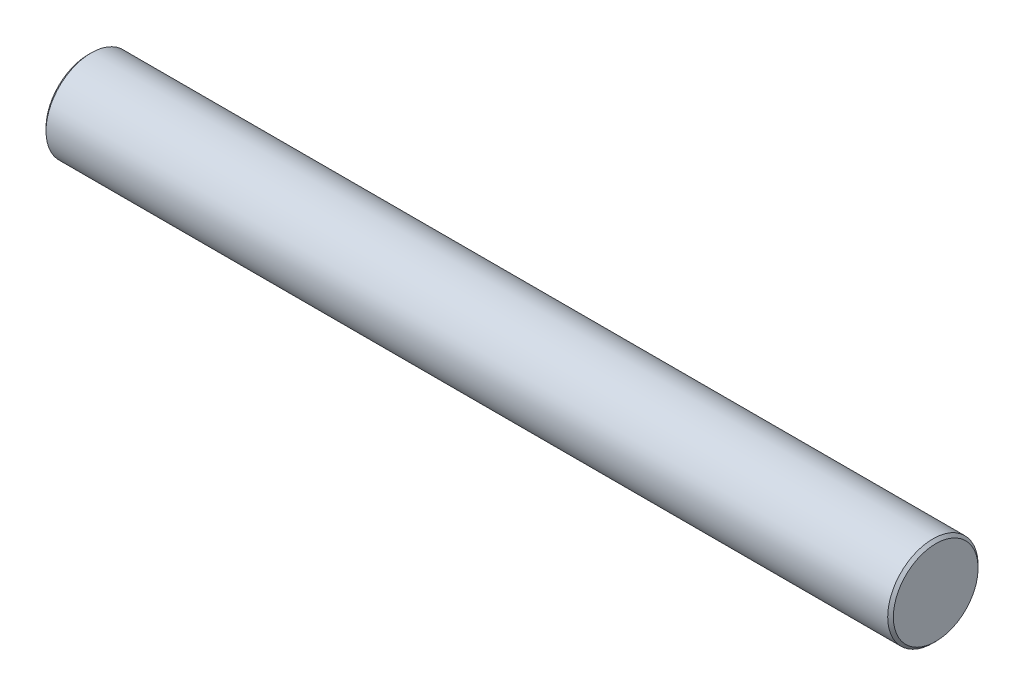
SolidWorks part; units mm, degrees
ref_plane "前视基准面" through (0, 0, 0) normal (0, 0, 1) x (1, 0, 0)
ref_plane "上视基准面" through (0, 0, 0) normal (0, 1, 0) x (1, 0, 0)
ref_plane "右视基准面" through (0, 0, 0) normal (1, 0, 0) x (0, 0, -1)
sketch "草图1" plane through (0, 0, 0) normal (0, 0, 1) x (1, 0, 0)
  line L0 (0, 0) -> (50000, 0) construction
  line L1 (0, 0) -> (0, 50000) construction
  line L3 (-75, 8) -> (75, 8)
  line L4 (-75, 8) -> (-75, 0)
  line L5 (-75, 0) -> (75, 0)
  line L6 (75, 8) -> (75, 0)
  dimension "D1" = 150
  dimension "D2" = 16
revolve "旋转1" add sketch "草图1" angle 360 about L0
chamfer "倒角1" distance 0.5 angle 45 2 edges at (75, 0, 8) (-75, 0, 8)
ref_plane "基准面1" through (0, 8, 0) normal (0, 1, 0) x (1, 0, 0)
ref_plane "基准面3" through (0, 0, 8) normal (0, 0, 1) x (1, 0, 0)
sketch "草图2" [suppressed] plane through (0, 10, 0) normal (0, 1, 0) x (1, 0, 0)
  line L0 (0, 0) -> (50000, 0) construction
  line L1 (64, 10) -> (-64, 10) construction
  line L2 (-55, -10) -> (-45, -10)
  line L3 (-55, -10) -> (-55, 10)
  line L4 (-55, 10) -> (-45, 10)
  line L5 (-45, -10) -> (-45, 10)
  line L6 (-55, -10) -> (-45, 10) construction
  line L7 (-55, 10) -> (-45, -10) construction
  line L8 (-65, 9) -> (-65, -9) construction
  point P3 (-50, 0)
  dimension "D1" = 10
  dimension "D2" = 10
  dimension "D3" = 10
extrude "切除-拉伸1" [suppressed] cut sketch "草图2" against normal blind 1
sketch "草图3" [suppressed] plane through (0, 10, 0) normal (0, 1, 0) x (1, 0, 0)
  line L0 (0, 0) -> (50000, 0) construction
  line L1 (64, 10) -> (-64, 10) construction
  line L2 (-52, -10) -> (-42, -10)
  line L3 (-52, -10) -> (-52, 10)
  line L4 (-52, 10) -> (-42, 10)
  line L5 (-42, -10) -> (-42, 10)
  line L6 (-52, -10) -> (-42, 10) construction
  line L7 (-52, 10) -> (-42, -10) construction
  line L8 (-65, 9) -> (-65, -9) construction
  line L9 (45, -10) -> (55, -10)
  line L10 (45, -10) -> (45, 10)
  line L11 (45, 10) -> (55, 10)
  line L12 (55, -10) -> (55, 10)
  line L13 (45, -10) -> (55, 10) construction
  line L14 (45, 10) -> (55, -10) construction
  line L15 (65, -9) -> (65, 9) construction
  point P3 (-47, 0)
  point P10 (50, 0)
  dimension "D1" = 10
  dimension "D2" = 10
  dimension "D3" = 13
  dimension "D4" = 10
  dimension "D5" = 20
extrude "切除-拉伸2" [suppressed] cut sketch "草图3" against normal blind 1
ref_plane "基准面2" through (-50, 0, 0) normal (-1, 0, 0) x (0, 0, 1)
sketch "草图4" [suppressed] plane through (-40, 0, 0) normal (-1, 0, 0) x (0, 0, 1)
  line L1 (-8.5, -10) -> (8.5, -10)
  line L2 (-8.5, -10) -> (-8.5, 10)
  line L3 (-8.5, 10) -> (8.5, 10)
  line L4 (8.5, -10) -> (8.5, 10)
  line L5 (-8.5, -10) -> (8.5, 10) construction
  line L6 (-8.5, 10) -> (8.5, -10) construction
  circle A0 centre (0, 0) radius 10 construction
  point P0 (0, 0)
  dimension "D1" = 14
extrude "切除-拉伸3" [suppressed] cut sketch "草图4" against normal blind 10 flip side to cut
sketch "草图8" plane through (0, 0, 8) normal (0, 0, -1) x (1, 0, 0)
  line L0 (0, 0) -> (50000, 0) construction
  line L1 (-67.5, 0) -> (-75, 0) construction
  line L2 (-75, 7.5) -> (-75, -7.5) construction
  line L3 (-67.5, -2.5) -> (-75, -2.5)
  line L4 (-67.5, 2.5) -> (-75, 2.5)
  line L5 (-75, 2.5) -> (-75, -2.5)
  arc A0 (-67.5, -2.5) -> (-67.5, 2.5) centre (-67.5, 0) ccw
  dimension "D1" = 5
  dimension "D2" = 10
extrude "切除-拉伸5" [suppressed] cut sketch "草图8" along normal blind 3
sketch "草图5" plane through (0, 0, 8) normal (0, 0, -1) x (1, 0, 0)
  line L0 (0, 0) -> (50000, 0) construction
  line L1 (-17.5, 0) -> (-12.5, 0) construction
  line L2 (-17.5, 2.5) -> (-12.5, 2.5)
  line L3 (-17.5, -2.5) -> (-12.5, -2.5)
  line L4 (-75, 7.5) -> (-75, -7.5) construction
  arc A0 (-17.5, 2.5) -> (-17.5, -2.5) centre (-17.5, 0) ccw
  arc A1 (-12.5, -2.5) -> (-12.5, 2.5) centre (-12.5, 0) ccw
  point P5 (-15, 0)
  dimension "D1" = 10
  dimension "D2" = 55
  dimension "D3" = 5
extrude "切除-拉伸4" [suppressed] cut sketch "草图5" along normal blind 3
sketch "草图6" [suppressed] plane through (0, 0, 0) normal (0, 0, 1) x (1, 0, 0)
  line L0 (-28, 10) -> (-25, 7)
  line L1 (64, 10) -> (-64, 10) construction
  line L2 (-25, 2.644) -> (-25, 50002.644) construction
  line L3 (-22, 10) -> (-25, 7)
  line L4 (-28, 10) -> (-22, 10)
  line L5 (-65, 9) -> (-65, -9) construction
  line L6 (0, 0) -> (50000, 0) construction
  dimension "D1" = 90
  dimension "D2" = 4
  dimension "D3" = 40
revolve "切除-旋转1" [suppressed] cut sketch "草图6" angle 360 about L6
sketch "草图7" [suppressed] plane through (0, 0, 0) normal (0, 0, 1) x (1, 0, 0)
  line L0 (-15, 0.2481) -> (-15, 50000.2481) construction
  line L1 (35, -0.0299) -> (35, 49999.9701) construction
  line L2 (0, 0) -> (50000, 0) construction
  line L3 (-18, 10) -> (-15, 7)
  line L4 (64, 10) -> (-64, 10) construction
  line L5 (32, 10) -> (35, 7)
  line L6 (-12, 10) -> (-15, 7)
  line L7 (38, 10) -> (35, 7)
  line L8 (-18, 10) -> (-12, 10)
  line L10 (32, 10) -> (38, 10)
  line L11 (-65, 9) -> (-65, -9) construction
  dimension "D1" = 90
  dimension "D2" = 90
  dimension "D3" = 4
  dimension "D4" = 4
  dimension "D5" = 50
  dimension "D6" = 50
revolve "切除-旋转2" [suppressed] cut sketch "草图7" angle 360 about L2
ref_plane "基准面4" [suppressed] through (-45, 0, 0) normal (-1, 0, 0) x (0, 0, 1)
ref_plane "基准面5" [suppressed] through (25, 0, 0) normal (1, 0, 0) x (0, 0, -1)
sketch "草图9" [suppressed] plane through (-45, 0, 0) normal (-1, 0, 0) x (0, 0, 1)
  line L1 (-8.5, -10) -> (8.5, -10)
  line L2 (-8.5, -10) -> (-8.5, 10)
  line L3 (-8.5, 10) -> (8.5, 10)
  line L4 (8.5, -10) -> (8.5, 10)
  line L5 (-8.5, -10) -> (8.5, 10) construction
  line L6 (-8.5, 10) -> (8.5, -10) construction
  circle A0 centre (0, 0) radius 10 construction
  point P0 (0, 0)
  dimension "D1" = 14
extrude "切除-拉伸6" [suppressed] cut sketch "草图9" against normal blind 10 flip side to cut
sketch "草图10" [suppressed] plane through (25, 0, 0) normal (1, 0, 0) x (0, 0, -1)
  line L1 (-8.5, -10) -> (8.5, -10)
  line L2 (-8.5, -10) -> (-8.5, 10)
  line L3 (-8.5, 10) -> (8.5, 10)
  line L4 (8.5, -10) -> (8.5, 10)
  line L5 (-8.5, -10) -> (8.5, 10) construction
  line L6 (-8.5, 10) -> (8.5, -10) construction
  circle A0 centre (0, 0) radius 10 construction
  point P0 (0, 0)
  dimension "D1" = 14
extrude "切除-拉伸7" [suppressed] cut sketch "草图10" against normal blind 10 flip side to cut
